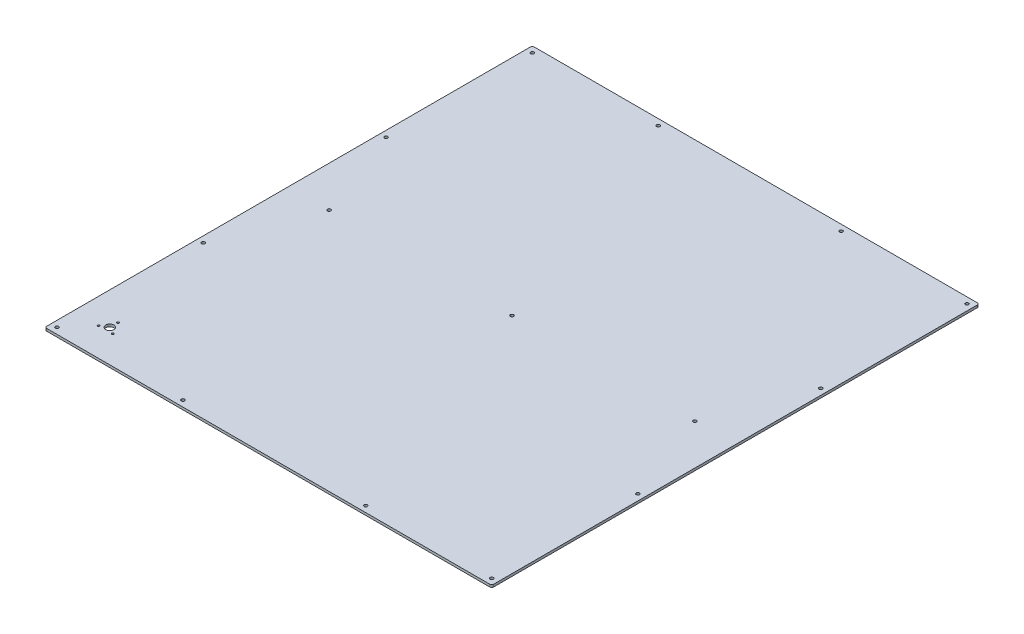
SolidWorks part; units mm, degrees
material "茶色亚克力"
ref_plane "前视基准面" through (0, 0, 0) normal (0, 0, 1) x (1, 0, 0)
ref_plane "上视基准面" through (0, 0, 0) normal (0, 1, 0) x (1, 0, 0)
ref_plane "右视基准面" through (0, 0, 0) normal (1, 0, 0) x (0, 0, -1)
sketch "草图1" plane through (0, 0, 0) normal (0, 1, 0) x (1, 0, 0)
  line L1 (-550, 600) -> (550, 600)
  line L2 (-550, 600) -> (-550, -600)
  line L3 (-550, -600) -> (550, -600)
  line L4 (550, 600) -> (550, -600)
  line L5 (-550, 600) -> (550, -600) construction
  line L6 (-550, -600) -> (550, 600) construction
  point P0 (0, 0)
  dimension "D1" = 1100
  dimension "D2" = 1200
extrude "凸台-拉伸1" add sketch "草图1" along normal blind 6
fillet "圆角1" radius 5 4 edges at (-550, 3, -600) (-550, 3, 600) (550, 3, -600) (550, 3, 600)
hole_wizard "Ø8.0 (8) 直径孔1" positions "草图2" profile "草图3" hole size "Ø8.0" standard "GB" end condition through all
sketch "草图2" plane through (0, 6, 0) normal (0, 1, 0) x (1, 0, 0)
  line L0 (-535, 585) -> (-535, -585) construction
  line L1 (-535, -585) -> (535, -585) construction
  line L4 (545, 600) -> (-545, 600) construction
  line L5 (-550, 595) -> (-550, -595) construction
  line L6 (0, -585) -> (0, 0) construction
  line L7 (0, 0) -> (-535, 0) construction
  point P0 (-535, 585)
  point P4 (535, 585)
  point P8 (-535, -585)
  point P12 (535, -585)
  point P34 (-225, -585)
  point P36 (225, -585)
  point P40 (0, 0)
  point P47 (-225, 585)
  point P49 (225, 585)
  point P53 (-535, -225)
  point P55 (-535, 225)
  point P57 (535, 225)
  point P59 (535, -225)
  point P68 (-450, 0)
  point P72 (450, 0)
  dimension "D1" = 15
  dimension "D2" = 15
  dimension "D3" = 450
  dimension "D4" = 450
  dimension "D5" = 900
sketch "草图3" plane through (-535, 6, -585) normal (1, 0, 0) x (0, 0, 1)
  line L0 (0, 0) -> (0, 6)
  line L1 (0, 6) -> (4, 6)
  line L2 (4, 6) -> (4, 0)
  line L5 (4, 0) -> (0, 0)
  line L11 (0, -6.35) -> (0, 107.95) construction
  dimension "通孔孔直径" = 8
  dimension "通孔孔深度" = 6
sketch "草图4" plane through (0, 6, 0) normal (0, 1, 0) x (1, 0, 0)
  line L0 (-545, -600) -> (545, -600) construction
  line L1 (-550, 595) -> (-550, -595) construction
  circle A0 centre (-470, -520) radius 10
  dimension "D1" = 80
  dimension "D3" = 20
  dimension "D2" = 80
extrude "切除-拉伸1" cut sketch "草图4" against normal through all
sketch "草图5" plane through (0, 6, 0) normal (0, 1, 0) x (1, 0, 0)
  line L0 (0, 975.3337) -> (0, 510) construction
  line L1 (60, 975.3337) -> (60, 510)
  line L2 (-60, 975.3337) -> (-60, 510)
  line L3 (0, 450) -> (109.9339, 450) construction
  line L4 (545, 600) -> (-545, 600) construction
  arc A0 (60, 975.3337) -> (-60, 975.3337) centre (0, 975.3337) ccw
  arc A1 (-60, 510) -> (60, 510) centre (0, 510) ccw
  point P2 (0, 742.6669)
  dimension "D1" = 120
  dimension "D2" = 150
extrude "切除-拉伸2" [suppressed] cut sketch "草图5" against normal through all
hole_wizard "Ø5.0 (5) 直径孔1" positions "草图8" profile "草图9" hole size "Ø5.0" standard "GB" end condition through all
sketch "草图8" plane through (0, 6, 0) normal (0, 1, 0) x (1, 0, 0)
  point P5 (-470, -499.7927)
  point P8 (-452.5, -530.1036)
  point P11 (-487.5, -530.1036)
sketch "草图9" plane through (-470, 6, 499.7927) normal (1, 0, 0) x (0, 0, 1)
  line L0 (0, 0) -> (0, 6)
  line L1 (0, 6) -> (2.5, 6)
  line L2 (2.5, 6) -> (2.5, 0)
  line L5 (2.5, 0) -> (0, 0)
  line L11 (0, -6.35) -> (0, 107.95) construction
  dimension "通孔孔直径" = 5
  dimension "通孔孔深度" = 6
